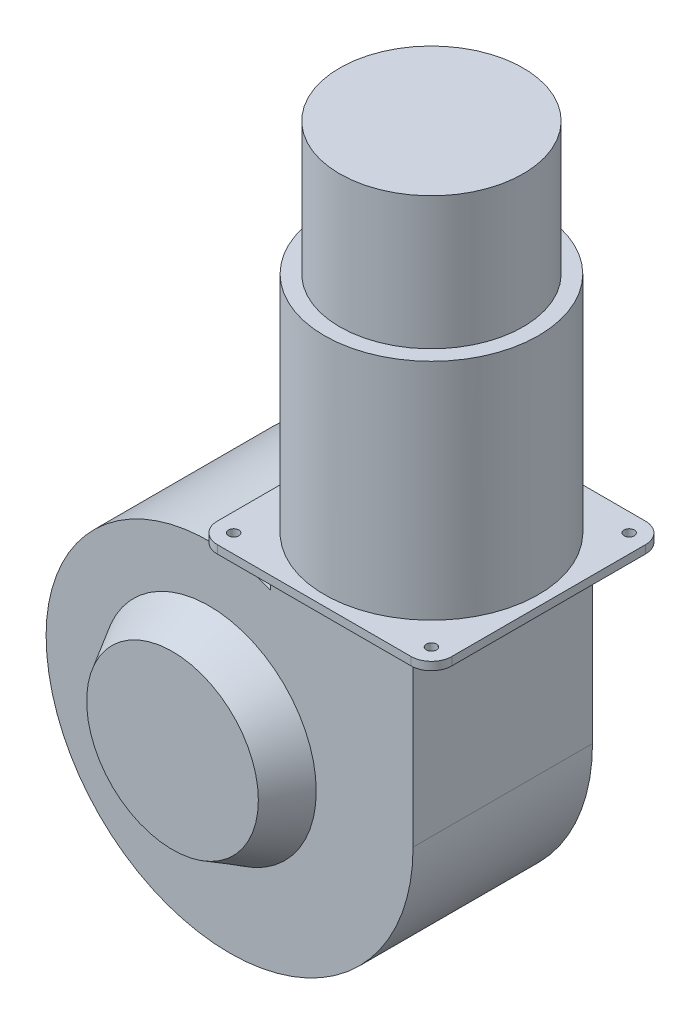
SolidWorks part; units mm, degrees
ref_plane "前视基准面" through (0, 0, 0) normal (0, 0, 1) x (1, 0, 0)
ref_plane "上视基准面" through (0, 0, 0) normal (0, 1, 0) x (1, 0, 0)
ref_plane "右视基准面" through (0, 0, 0) normal (1, 0, 0) x (0, 0, -1)
sketch "草图1" plane through (0, 0, 0) normal (0, 0, 1) x (1, 0, 0)
  line L0 (100, 0) -> (100, 90)
  line L1 (0, 0) -> (157.9154, 0) construction
  line L2 (30, 90) -> (30, 74.162)
  line L3 (30, 90) -> (100, 90)
  arc A0 (30, 74.162) -> (-80, 0) centre (0, 0) ccw
  arc A1 (-80, 0) -> (100, 0) centre (10, 0) ccw
  dimension "D1" = 160
  dimension "D2" = 100
  dimension "D3" = 70
  dimension "D4" = 90
  dimension "D5" = 90
extrude "凸台-拉伸1" add sketch "草图1" along normal blind 88
sketch "草图2" plane through (0, 0, 88) normal (0, 0, 1) x (1, 0, 0)
  circle A0 centre (0, 0) radius 52.5
  dimension "D1" = 105
extrude "凸台-拉伸2" add sketch "草图2" along normal blind 18 draft 30
sketch "草图3" plane through (0, 90, 0) normal (0, 1, 0) x (1, 0, 0)
  line L0 (100, -44) -> (-6.0324, -44) construction
  line L1 (100, -88) -> (100, 0) construction
  line L2 (65, 0) -> (65, -117.7426) construction
  line L3 (100, 0) -> (30, 0) construction
  line L5 (17.5, 13.5) -> (112.5, 13.5)
  line L6 (7.5, 3.5) -> (7.5, -91.5)
  line L7 (17.5, -101.5) -> (112.5, -101.5)
  line L8 (122.5, 3.5) -> (122.5, -91.5)
  arc A0 (112.5, 13.5) -> (122.5, 3.5) centre (112.5, 3.5) cw
  arc A1 (122.5, -91.5) -> (112.5, -101.5) centre (112.5, -91.5) cw
  arc A2 (17.5, -101.5) -> (7.5, -91.5) centre (17.5, -91.5) cw
  arc A3 (7.5, 3.5) -> (17.5, 13.5) centre (17.5, 3.5) cw
  circle A4 centre (16.5, 4.5) radius 2.5
  circle A5 centre (16.5, -92.5) radius 2.5
  circle A6 centre (113.5, -92.5) radius 2.5
  circle A7 centre (113.5, 4.5) radius 2.5
  point P14 (122.5, 13.5)
  point P17 (122.5, -101.5)
  point P22 (7.5, 13.5)
  dimension "D5" = 10
  dimension "D8" = 5
  dimension "D1" = 115
  dimension "D2" = 115
  dimension "D3" = 57.5
  dimension "D4" = 57.5
  dimension "D6" = 48.5
  dimension "D7" = 48.5
extrude "凸台-拉伸3" add sketch "草图3" along normal blind 4
sketch "草图4" plane through (0, 94, 0) normal (0, 1, 0) x (1, 0, 0)
  line L0 (65, 13.5) -> (65, -123.7646) construction
  line L1 (112.5, 13.5) -> (17.5, 13.5) construction
  line L2 (122.5, -44) -> (-19.8957, -44) construction
  line L3 (122.5, -91.5) -> (122.5, 3.5) construction
  circle A0 centre (65, -44) radius 52.5
  dimension "D1" = 105
extrude "凸台-拉伸4" add sketch "草图4" along normal blind 110
sketch "草图5" plane through (0, 204, 0) normal (0, 1, 0) x (1, 0, 0)
  circle A0 centre (65, -44) radius 45
  dimension "D1" = 90
extrude "凸台-拉伸5" add sketch "草图5" along normal blind 65
ref_plane "基准面1" through (20, 0, 0) normal (-1, 0, 0) x (0, 0, 1)
sketch "草图6" plane through (20, 0, 0) normal (-1, 0, 0) x (0, 0, 1)
  line L0 (44, 269) -> (44, 126.4825) construction
  line L1 (89, 269) -> (-1, 269) construction
  line L2 (96.5, 204) -> (-8.5, 204) construction
  line L3 (44, 239) -> (39.6699, 236.5)
  line L4 (39.6699, 236.5) -> (39.6699, 231.5)
  line L5 (39.6699, 231.5) -> (44, 229)
  line L6 (44, 229) -> (48.3301, 231.5)
  line L7 (48.3301, 231.5) -> (48.3301, 236.5)
  line L8 (48.3301, 236.5) -> (44, 239)
  circle A0 centre (44, 234) radius 5 construction
  dimension "D1" = 10
  dimension "D2" = 30
extrude "凸台-拉伸6" add sketch "草图6" along normal blind 5 and the other way blind 5 separate body
sketch "草图7" plane through (15, 0, 0) normal (-1, 0, 0) x (0, 0, 1)
  line L0 (96.5, 204) -> (-8.5, 204) construction
  circle A0 centre (44, 234) radius 4
  dimension "D1" = 8
  dimension "D2" = 30
extrude "凸台-拉伸7" add sketch "草图7" along normal blind 8
